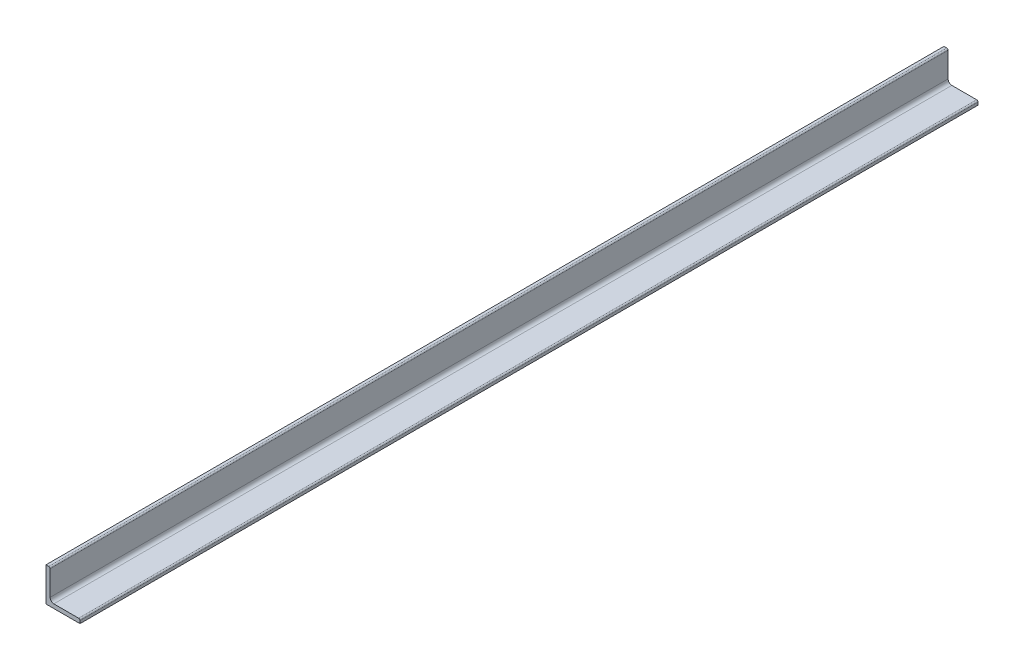
from build123d import *

# Parameters (mm, degrees)
BOSS_EXTRUDE1_DEPTH = 660.4


with BuildPart() as part:
    # Sketch1 → Boss-Extrude1 (new, symmetric)
    with BuildSketch(Plane.XY):
        with BuildLine():
            Line((0, 50), (0, 0))
            Line((0, 0), (50, 0))
            Line((50, 0), (50, 4))
            ThreePointArc((50, 4), (49.414213562, 5.414213562), (48, 6))
            Line((48, 6), (11.5, 6))
            ThreePointArc((11.5, 6), (7.610912703, 7.610912703), (6, 11.5))
            Line((6, 11.5), (6, 48))
            ThreePointArc((6, 48), (5.414213562, 49.414213562), (4, 50))
            Line((4, 50), (0, 50))
        make_face()
    extrude(amount=BOSS_EXTRUDE1_DEPTH, both=True)


solid = part.part
